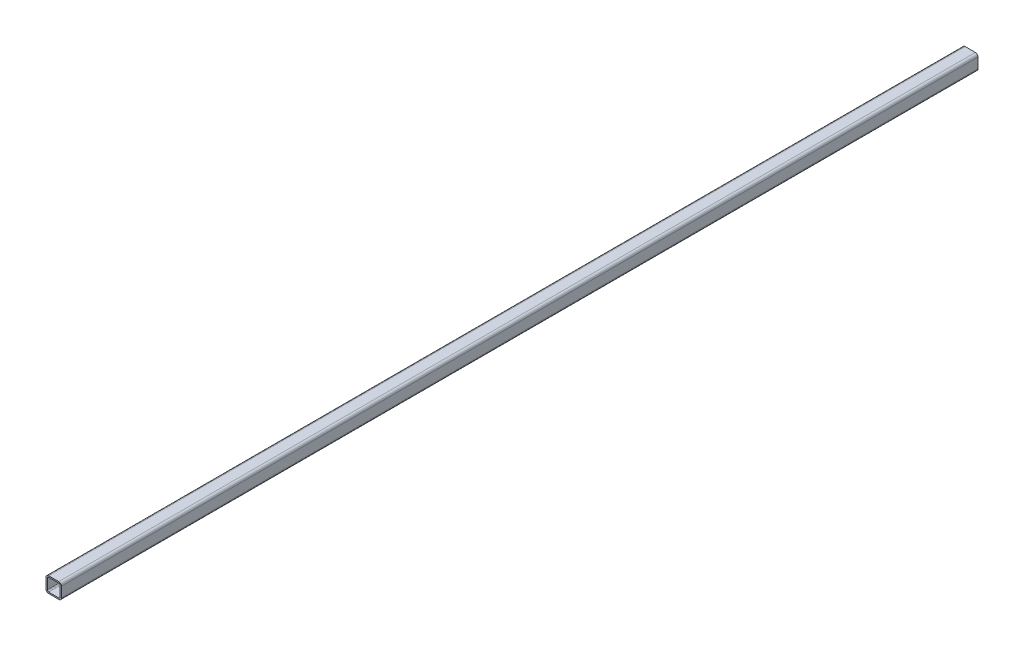
from build123d import *

# Parameters (mm, degrees)
BOSS_EXTRUDE1_DEPTH = 4160


with BuildPart() as part:
    # Sketch1 → Boss-Extrude1 (new body)
    with BuildSketch(Plane.XY):
        with BuildLine():
            Line((12, 0), (58, 0))
            ThreePointArc((58, 0), (66.485281374, 3.514718626), (70, 12))
            Line((70, 12), (70, 58))
            ThreePointArc((70, 58), (66.485281374, 66.485281374), (58, 70))
            Line((58, 70), (12, 70))
            ThreePointArc((12, 70), (3.514718626, 66.485281374), (0, 58))
            Line((0, 58), (0, 12))
            ThreePointArc((0, 12), (3.514718626, 3.514718626), (12, 0))
        make_face()
        with BuildLine():
            Line((12, 6), (58, 6))
            ThreePointArc((58, 6), (62.242640687, 7.757359313), (64, 12))
            Line((64, 12), (64, 58))
            ThreePointArc((64, 58), (62.242640687, 62.242640687), (58, 64))
            Line((58, 64), (12, 64))
            ThreePointArc((12, 64), (7.757359313, 62.242640687), (6, 58))
            Line((6, 58), (6, 12))
            ThreePointArc((6, 12), (7.757359313, 7.757359313), (12, 6))
        make_face(mode=Mode.SUBTRACT)
    extrude(amount=BOSS_EXTRUDE1_DEPTH)


solid = part.part
